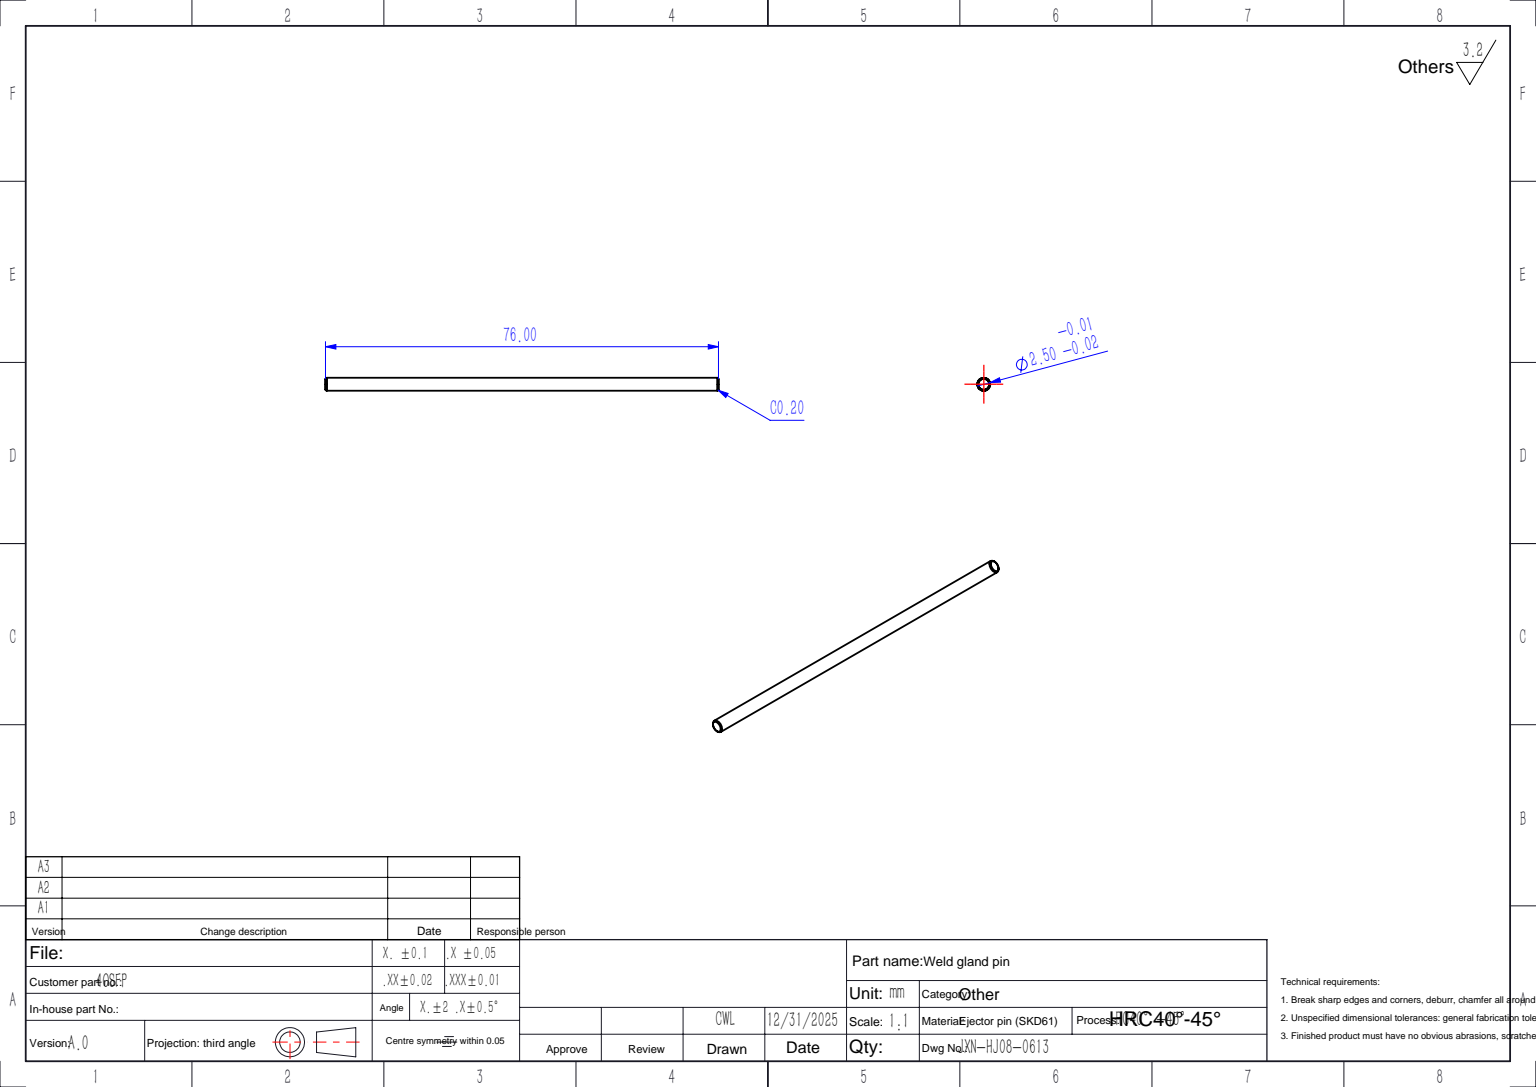
from build123d import *

# Parameters (mm, degrees)
SKETCH_1_R      = 1.25
EXTRUDE_1_DEPTH = 76
CHAMFER_1_SIZE  = 0.2


with BuildPart() as part:
    # 草图1 → 凸台-拉伸1 (new body)
    with BuildSketch(Plane(origin=(0, 0, 0), x_dir=(1, 0, 0), z_dir=(0, 1, 0))):
        with Locations(Location((0, 0, 0), (0, 0, 270))):
            Circle(SKETCH_1_R)
    extrude(amount=EXTRUDE_1_DEPTH)

    # 倒角1
    chamfer_1_edges = [part.edges().sort_by_distance(p)[0] for p in [
        (0, 0, -1.25),
        (0, 76, -1.25),
    ]]
    chamfer(chamfer_1_edges, length=CHAMFER_1_SIZE)


solid = part.part
